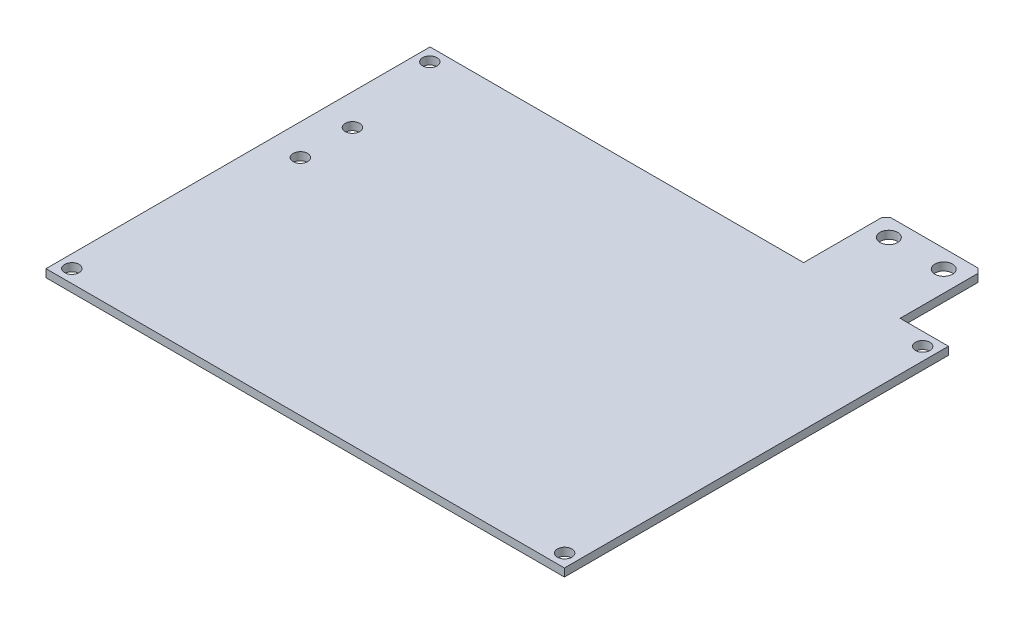
from build123d import *

# Parameters (mm, degrees)
SKETCH_1_R      = 1.55
SKETCH_1_R_2    = 1.9
EXTRUDE_1_DEPTH = 1.7


with BuildPart() as part:
    # 草图1 → 凸台-拉伸1 (new body)
    with BuildSketch(Plane(origin=(0, 0, 0), x_dir=(1, 0, 0), z_dir=(0, 1, 0))):
        Polygon((-55.75, -41.3), (55.75, -41.3), (55.75, 41.3), (45.35, 41.3), (45.35, 58.05), (44.35, 59.05), (25.6, 59.05), (24.6, 58.05), (24.6, 41.3), (-55.75, 41.3), align=None)
        with Locations(Location((-53, 38.5, 0), (0, 0, 270))):
            Circle(SKETCH_1_R, mode=Mode.SUBTRACT)
        with Locations(Location((53, 38.5, 0), (0, 0, 90))):
            Circle(SKETCH_1_R, mode=Mode.SUBTRACT)
        with Locations(Location((53, -38.5, 0), (0, 0, 270))):
            Circle(SKETCH_1_R, mode=Mode.SUBTRACT)
        with Locations(Location((-53, -38.5, 0), (0, 0, 90))):
            Circle(SKETCH_1_R, mode=Mode.SUBTRACT)
        with Locations(Location((29.075, 55.15, 0), (0, 0, 270))):
            Circle(SKETCH_1_R_2, mode=Mode.SUBTRACT)
        with Locations(Location((40.875, 55.15, 0), (0, 0, 90))):
            Circle(SKETCH_1_R_2, mode=Mode.SUBTRACT)
        with Locations(Location((-49.1, 17.95, 0), (0, 0, 270))):
            Circle(SKETCH_1_R, mode=Mode.SUBTRACT)
        with Locations(Location((-49.1, 6.75, 0), (0, 0, 270))):
            Circle(SKETCH_1_R, mode=Mode.SUBTRACT)
    extrude(amount=EXTRUDE_1_DEPTH)


solid = part.part
